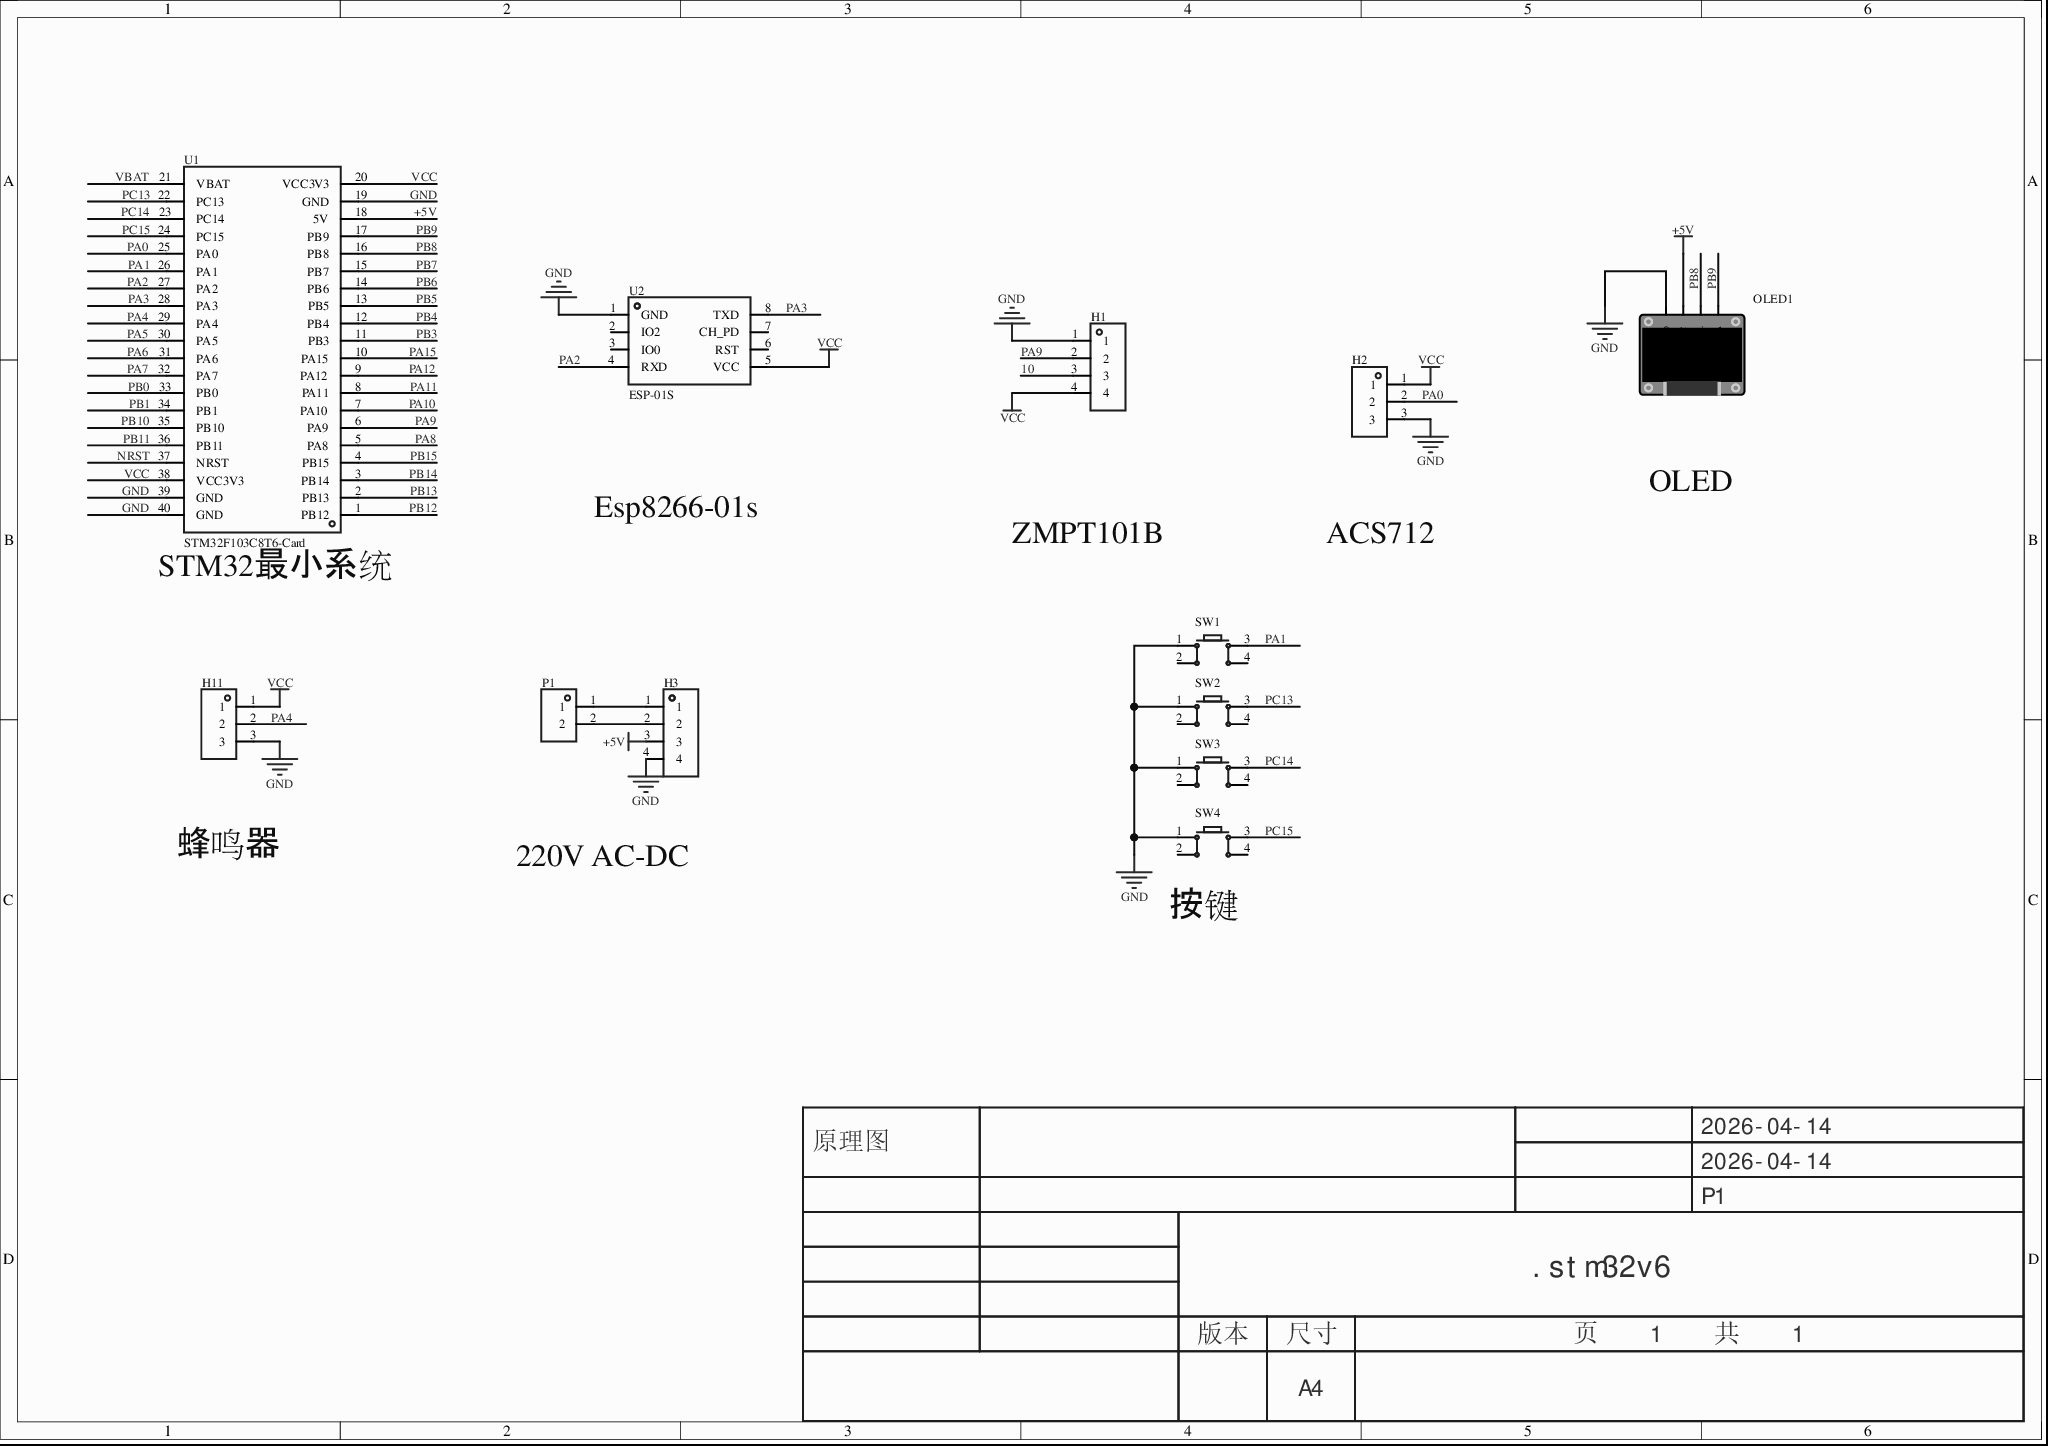
[diagram p0: MISC51329-3.schdoc]
# Altium project MISC51329-2.PrjPcb
1 sheet, 12 parts. Net scope: global (net labels, ports and power ports of the same name join across sheets).
Board file: MISC51329.pcbdoc

## Sheet MISC51329-3.schdoc
size 297 x 209 mm; Version: V1.0; @Project Name: MISC51329; @Page Count: 1; @Update Date: 2026-04-14; @Create Date: 2026-04-14; @Schematic Name: MISC51329; @Page No: 1; @Create Time: 23:22:16; @Update Time: 17:32:40; @Board Name: MISC51329

### Parts
H1  (no value)  [HDR-TH_4P-P2.54-V-M]
H2  (no value)  [HDR-TH_3P-P2.54-V-F]
H3  (no value)  [HDR-TH_4P-P2.54-V-F]
H11  (no value)  [HDR-TH_3P-P2.54-V-F]
OLED1  (no value)  [0.96OLED_4P]
P1  KF301-2P接线端子  [CONN-TH_XY301V-A-5.0-2P]  (value not drawn)
SW1  (no value)  [SW-TH_4P-L6.0-W6.0-P4.50-LS6.5]
SW2  (no value)  [SW-TH_4P-L6.0-W6.0-P4.50-LS6.5]
SW3  (no value)  [SW-TH_4P-L6.0-W6.0-P4.50-LS6.5]
SW4  (no value)  [SW-TH_4P-L6.0-W6.0-P4.50-LS6.5]
U1  STM32F103C8T6-Card  [CONN-TH_L53.3-W22.9_STM32F103C8T6-CARD]
U2  ESP-01S  [WIFIM-TH_ESP-01S]

### Nets
+5V: H3.3 OLED1.2(VCC) U1.18(5V)
GND: H1.1 H2.3 H3.4 H11.3 OLED1.1(GND) SW1.1 SW2.1 SW3.1 SW4.1 U1.19(GND) U1.39(GND) U1.40(GND) U2.1(GND)
VCC: H1.4 H2.1 H11.1 U1.20(VCC3V3) U1.38(VCC3V3) U2.5(VCC)
10: H1.3
NRST: U1.37(NRST)
PA0: H2.2 U1.25(PA0)
PA1: SW1.3 U1.26(PA1)
PA2: U1.27(PA2) U2.4(RXD)
PA3: U1.28(PA3) U2.8(TXD)
PA4: H11.2 U1.29(PA4)
PA5: U1.30(PA5)
PA6: U1.31(PA6)
PA7: U1.32(PA7)
PA8: U1.5(PA8)
PA9: H1.2 U1.6(PA9)
PA10: U1.7(PA10)
PA11: U1.8(PA11)
PA12: U1.9(PA12)
PA15: U1.10(PA15)
PB0: U1.33(PB0)
PB1: U1.34(PB1)
PB3: U1.11(PB3)
PB4: U1.12(PB4)
PB5: U1.13(PB5)
PB6: U1.14(PB6)
PB7: U1.15(PB7)
PB8: OLED1.3(SCL) U1.16(PB8)
PB9: OLED1.4(SDA) U1.17(PB9)
PB10: U1.35(PB10)
PB11: U1.36(PB11)
PB12: U1.1(PB12)
PB13: U1.2(PB13)
PB14: U1.3(PB14)
PB15: U1.4(PB15)
PC13: SW2.3 U1.22(PC13)
PC14: SW3.3 U1.23(PC14)
PC15: SW4.3 U1.24(PC15)
VBAT: U1.21(VBAT)
NetH3_1: H3.1 P1.1
NetH3_2: H3.2 P1.2

Not connected (* = marked no-connect by the designer): SW1 2 4; SW2 2 4; SW3 2 4; SW4 2 4; U2 2(IO2)* 3(IO0)* 6(RST)* 7(CH_PD)*

### Notes on the sheet
- Esp8266-01s
- OLED
- (near U1) STM32最小系统
- ZMPT101B
- ACS712
- 蜂鸣器
- 220V AC-DC
- (near SW4) 按键
- Labels drawn without touching a wire or pin: VCC
- 2026-04-14
- 原理图
- P1
- .stm32v6
- 版本
- 尺寸
- A4
- 页    1    共    1

### Library data of the parts
H1 = HDR-M_2.54_1x4P: Symbol: PZ254V-11-04P; ConvertToPcb: yes; ModelId: 112f4d05e8d64e99ab9a333894bea4f90819f05c4eef4c71ace90d822a990e87; ModelName: HDR-TH_4P-P2.54-M-LI-1X4P; ModelTransform: 399.999,104.7242,0,0,0,0,0,0,-118.11; Device: HDR-M_2.54_1x4P; AddInBom: yes; SupplierPart: C492403; Supplier Footprint: 插件; FootprintName: HDR-TH_4P-P2.54-V-M
H2 H11 = HDR-F_2.54_1x3P: Symbol: PM254V-11-03-H85; 3D Model: f3b3cc5aae9641bf9e56fc160cef875b; 3D Model Transform: 299.9994,100,0,0,0,0,0,0,-118.11; ConvertToPcb: yes; ModelName: HDR2.54-F-LI-1X3P; Device: HDR-F_2.54_1x3P; Supplier Part: C541850; Supplier Footprint: 插件; AddInBom: yes; FootprintName: HDR-TH_3P-P2.54-V-F
H3 = HDR-F_2.54_1x4P: Symbol: 2.54-1*4P母; ConvertToPcb: yes; ModelId: d187812051054f85879fcaa51a310d8e0819f05c4eef4c71ace90d822a990e87; ModelTransform: 419.6842,98.464,0,0,0,0,0,0,-118.11; Device: HDR-F_2.54_1x4P; AddInBom: yes; SupplierPart: C2718488; Supplier Footprint: 插件; FootprintName: HDR-TH_4P-P2.54-V-F; ModelName: HDR-TH_4P-P2.54-V-F
OLED1 = 0.96OLED模块_4P: ConvertToPcb: yes; ModelId: 79c000fdb68d45a296c2e9bedf4f9055; ModelTransform: 1393.69792,1318.895,0,0,0,0,0,-560.079,-137.795; Symbol: 0.96OLED模块_4P; Device: 0.96OLED模块_4P; AddInBom: yes; FootprintName: 0.96OLED_4P; Supplier Footprint: 插件; ModelName: 0.96OLED_4P
P1 = KF301-2P接线端子: AddInBom: yes; ModelId: ef7ead88b0f2448d904975b26718870f; ModelTransform: 417.322,299.212,0,0,0,0,11.811,-7.835,-157.48; Symbol: KF301-2P接线端子; Device: KF301-2P接线端子; LCSC Part Name: KF301-2P接线端子; SupplierPart: C9900016950; ManufacturerPart: KF301-2P接线端子; Supplier Footprint: CK301-2P; Supplier: LCSC; ConvertToPcb: yes; FootprintName: CONN-TH_XY301V-A-5.0-2P; ModelName: CONN-TH_XY301V-A-5.0-2P
SW1-SW4 = Key_TH_6x6x6: 触点电流:50mA;额定电压(DC):12V;绝缘电阻:100MΩ;电路结构:单刀单掷;安装方式:直插;按钮形状:圆形按钮;按钮/盖帽颜色:黑色;作用力:260gf@±30gf;工作温度:-25℃~+70℃;引脚样式:PC引脚;开关长度:6mm;开关宽度:6mm;开关高度:6mm;带支架:否;; Symbol: 轻触按键; AddInBom: yes; ModelId: 20eee248bc684ccd8cbdbb1d0d91ec6f0819f05c4eef4c71ace90d822a990e87; ModelName: SW-TH_4P-L6.0-W6.0-H5.0-LS6.5-P4.50; ModelTransform: 236.22,323.03,0,90,0,0,0,0,-137.795; Device: Key_TH_6x6x6; ConvertToPcb: yes; FootprintName: SW-TH_4P-L6.0-W6.0-P4.50-LS6.5; Supplier Footprint: 插件
U1 = STM32F103C8T6-Card: AddInBom: yes; Symbol: STM32F103C8T6-CARD; Device: STM32F103C8T6-Card; LCSC Part Name: STM32F103C8T6-Card; SupplierPart: C9900077949; ManufacturerPart: STM32F103C8T6-Card; Supplier Footprint: 插件; Supplier: LCSC; ConvertToPcb: yes; FootprintName: CONN-TH_L53.3-W22.9_STM32F103C8T6-CARD
U2 = ESP-01S_C111009: 3D Model: eb7175da78ae48b3b1568cfe3027405f0819f05c4eef4c71ace90d822a990e87; 3D Model Transform: 582.676,976.37608,0,0,0,0,0,388.346,-118.11; AddInBom: yes; Symbol: ESP-01S; Device: ESP-01S_C111009; LCSC Part Name: ESP-01S; Supplier Part: C111009; Manufacturer Part: ESP-01S; Supplier Footprint: -; JLCPCB Part Class: Extended Part; Supplier: LCSC; ConvertToPcb: yes; FootprintName: WIFIM-TH_ESP-01S; ModelName: WIFIM-TH_ESP-01S